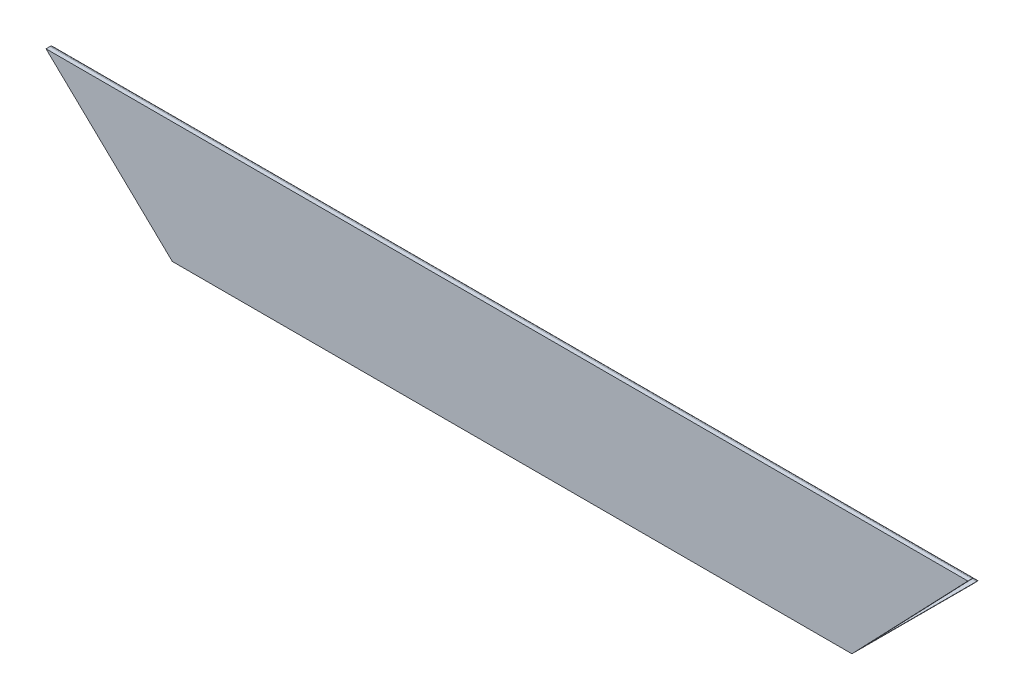
from build123d import *

# Parameters (mm, degrees)
EXTRUDE1_DEPTH    = 900
SKETCH2_OUTSIDE_W = 2163.11
SKETCH2_OUTSIDE_H = 463.11
EXTRUDE5_DEPTH    = 100


with BuildPart() as part:
    # Sketch1 → Extrude1 (new, symmetric)
    with BuildSketch(Plane(origin=(0, 0, 0), x_dir=(0, 0, -1), z_dir=(1, 0, 0))):
        with BuildLine():
            Line((-44, 47.3), (-44, -32))
            ThreePointArc((-44, -32), (-40.485281374, -40.485281374), (-32, -44))
            Line((-32, -44), (47.3, -44))
            ThreePointArc((47.3, -44), (49.209188309, -44.790811691), (50, -46.7))
            Line((50, -46.7), (50, -50))
            Line((50, -50), (-50, -50))
            Line((-50, -50), (-50, 50))
            Line((-50, 50), (-46.7, 50))
            ThreePointArc((-46.7, 50), (-44.790811691, 49.209188309), (-44, 47.3))
        make_face()
    extrude(amount=EXTRUDE1_DEPTH, both=True)

    # Sketch2 outside → Extrude5 (cut)
    with BuildSketch(Plane.XY.offset(50)):
        Rectangle(SKETCH2_OUTSIDE_W, SKETCH2_OUTSIDE_H)
        Polygon((-138.272358385, 50), (-900, 50), (-502.876430533, -330.516583835), align=None, mode=Mode.SUBTRACT)
    extrude(amount=-EXTRUDE5_DEPTH, mode=Mode.SUBTRACT)


solid = part.part
